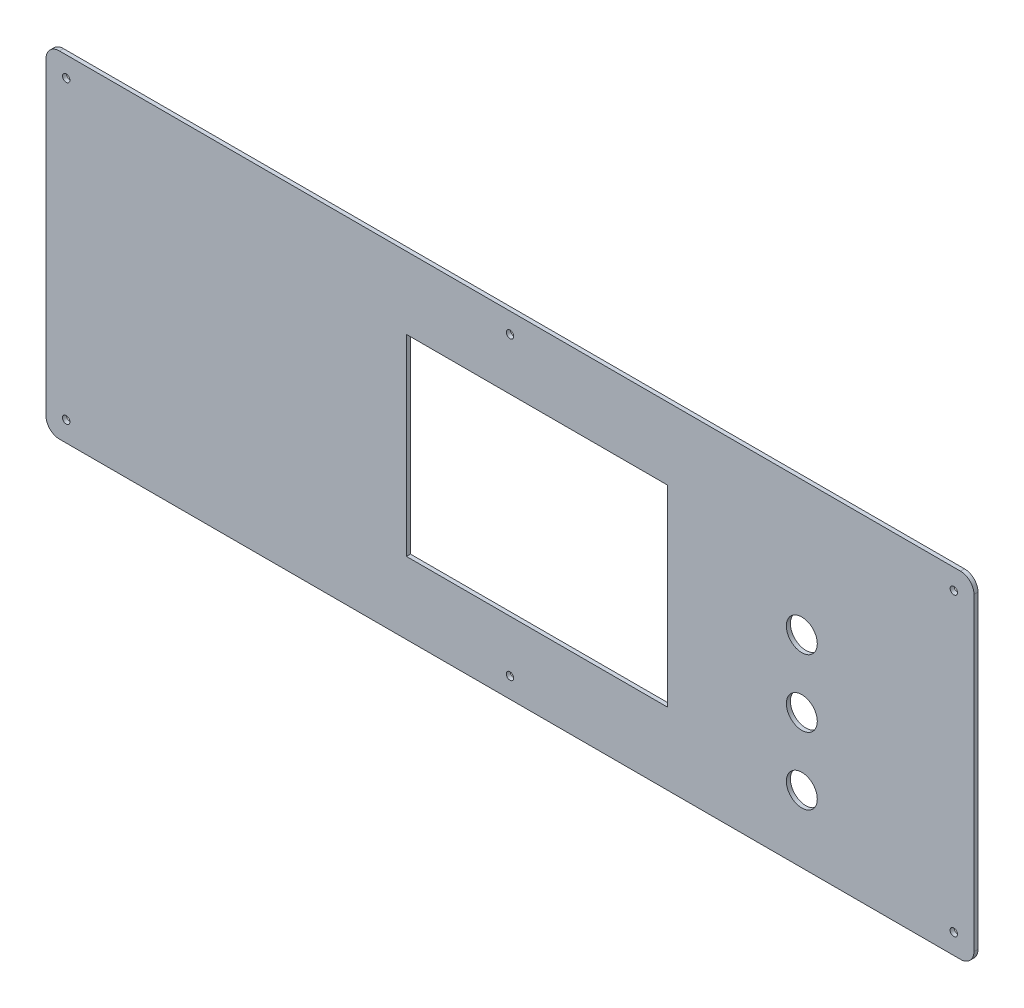
from build123d import *

# Parameters (mm, degrees)
SKETCH_1_W                  = 690
SKETCH_1_H                  = 250
EXTRUDE_1_DEPTH             = 1.5
SKETCH_2_W                  = 194
SKETCH_2_H                  = 143
CUT_EXTRUDE_1_DEPTH         = 6
SKETCH_3_R                  = 11.5
CUT_EXTRUDE_2_DEPTH         = 6
FILLET_1_R                  = 10
HOLE_WIZARD_5_5_5_5_1_D     = 5.5
HOLE_WIZARD_5_5_5_5_1_DEPTH = 10
HOLE_WIZARD_5_5_5_5_1_TIP   = 1.652366702


with BuildPart() as part:
    # 草图1 → 凸台-拉伸1 (new, symmetric)
    with BuildSketch(Plane.XY):
        Rectangle(SKETCH_1_W, SKETCH_1_H)
    extrude(amount=EXTRUDE_1_DEPTH, both=True)

    # 草图2 → 切除-拉伸1 (cut)
    with BuildSketch(Plane.XY.offset(1.5)):
        with Locations((20, 0)):
            Rectangle(SKETCH_2_W, SKETCH_2_H)
    extrude(amount=-CUT_EXTRUDE_1_DEPTH, mode=Mode.SUBTRACT)

    # 草图3 → 切除-拉伸2 (cut)
    with BuildSketch(Plane.XY.offset(1.5)):
        with Locations((217, -25)):
            Circle(SKETCH_3_R)
        with Locations((217, -75)):
            Circle(SKETCH_3_R)
        with BuildLine():
            ThreePointArc((205.992928436, 28.33082206), (219.353810017, 13.74346508), (225.750187968, 32.462185372))
            ThreePointArc((225.750187968, 32.462185372), (214.646189983, 36.25653492), (205.992928436, 28.33082206))
        make_face()
    extrude(amount=-CUT_EXTRUDE_2_DEPTH, mode=Mode.SUBTRACT)

    # 圆角1
    fillet_1_edges = [part.edges().sort_by_distance(p)[0] for p in [
        (345, -125, 0),
        (-345, -125, 0),
        (-345, 125, 0),
        (345, 125, 0),
    ]]
    fillet(fillet_1_edges, radius=FILLET_1_R)

    # Ø5.5 (5.5) 直径孔1
    with Locations(Plane.XY.offset(1.5)):
        with Locations((-330, 110), (0, 110), (330, 110), (330, -110), (0, -110), (-330, -110)):
            Hole(HOLE_WIZARD_5_5_5_5_1_D / 2, depth=HOLE_WIZARD_5_5_5_5_1_DEPTH)
            with Locations((0, 0, -(HOLE_WIZARD_5_5_5_5_1_DEPTH + HOLE_WIZARD_5_5_5_5_1_TIP / 2))):  # 118° drill point
                Cone(0, HOLE_WIZARD_5_5_5_5_1_D / 2, HOLE_WIZARD_5_5_5_5_1_TIP, mode=Mode.SUBTRACT)


solid = part.part
